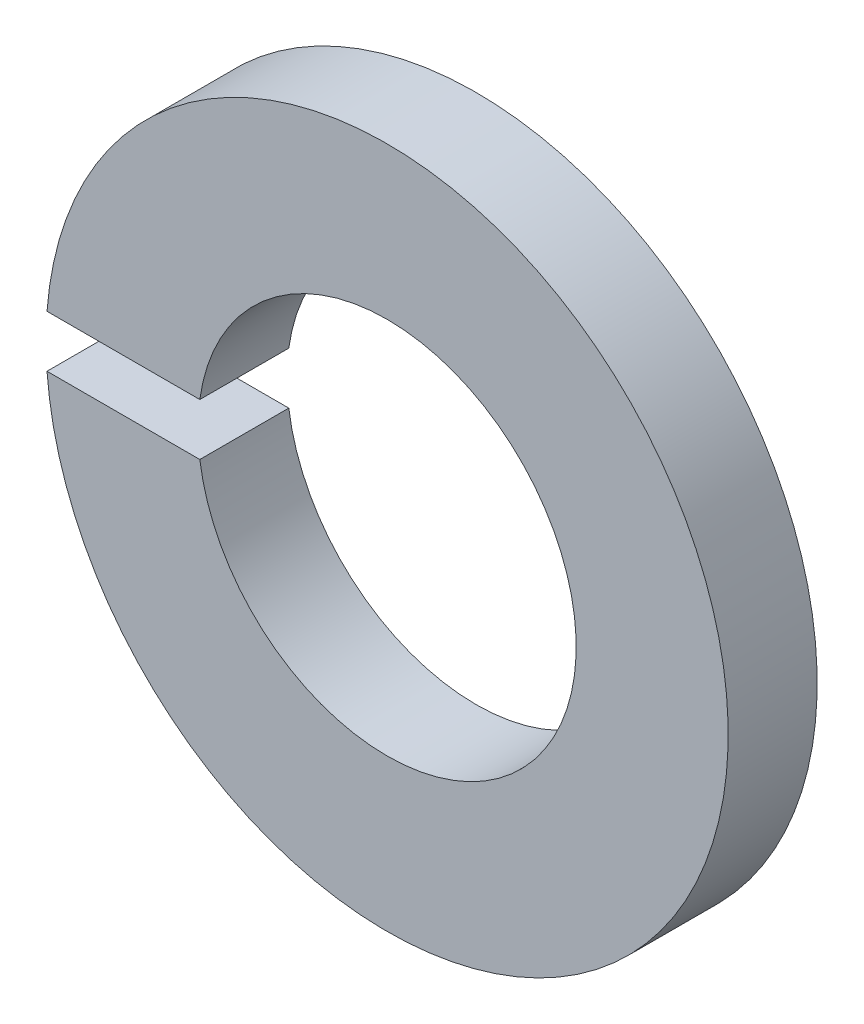
SolidWorks part; units mm, degrees
ref_plane "前视基准面" through (0, 0, 0) normal (0, 0, 1) x (1, 0, 0)
ref_plane "上视基准面" through (0, 0, 0) normal (0, 1, 0) x (1, 0, 0)
ref_plane "右视基准面" through (0, 0, 0) normal (1, 0, 0) x (0, 0, -1)
ref_plane "基准面1" through (0, 0, 1.2) normal (0, 0, 1) x (1, 0, 0)
sketch "草图1" plane through (0, 0, 1.2) normal (0, 0, 1) x (1, 0, 0)
  line L0 (-4.5867, 0.35) -> (-2.5259, 0.35)
  line L1 (-2.5259, -0.35) -> (-4.5867, -0.35)
  arc A0 (-2.5259, 0.35) -> (-2.5259, -0.35) centre (0, 0) cw
  arc A1 (-4.5867, -0.35) -> (-4.5867, 0.35) centre (0, 0) ccw
extrude "凸台-拉伸1" add sketch "草图1" against normal blind 1.2
